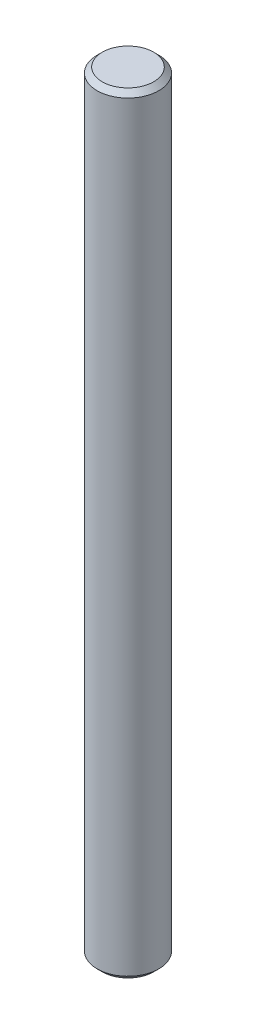
SolidWorks part; units mm, degrees
ref_plane "Front Plane" through (0, 0, 0) normal (0, 0, 1) x (1, 0, 0)
ref_plane "Top Plane" through (0, 0, 0) normal (0, 1, 0) x (1, 0, 0)
ref_plane "Right Plane" through (0, 0, 0) normal (1, 0, 0) x (0, 0, -1)
sketch "Sketch1" plane through (0, 0, 0) normal (0, 1, 0) x (1, 0, 0)
  circle A0 centre (0, 0) radius 0.6
  dimension "D1" = 1.2
extrude "Boss-Extrude1" add sketch "Sketch1" along normal blind 15
chamfer "Chamfer1" distance 0.1 angle 45 2 edges at (0, 0, 0.6) (0, 15, 0.6)
